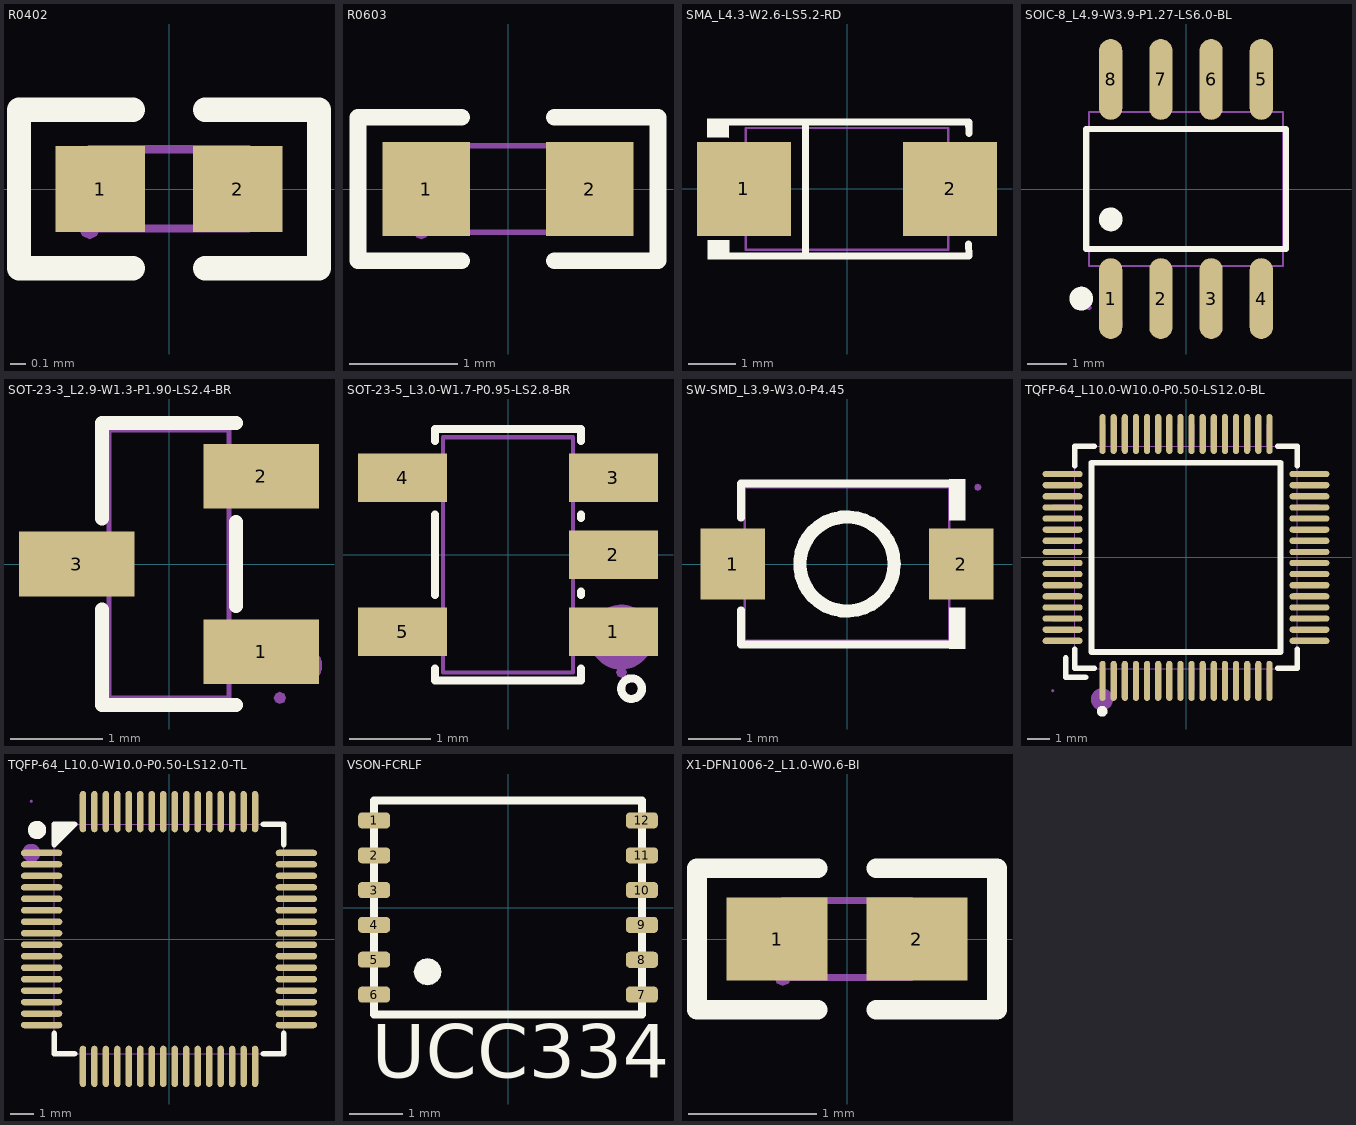
[diagram p0: the footprints below, top view; thin cyan lines are the x and y axes]
# Altium footprint library MISC86293-39.PcbLib: 27 footprints (part 2 of 2)
Each footprint in its own frame and in the unit in brackets; x right, y up, seen from the top. Pads: shape width x height; smd on the part's side, far side on the other; paste and mask are expansions set on the pad; w line width, h text height; cw(c..) or ccw(c..) is an arc to the next point about the centre after c.

## R0402 [mm]
pads (2):
  rect 0.566x0.54 smd paste-100 mask+0.051: 1(-0.433,0) 2(0.433,0)
Top Overlay:
  lines w0.152: -0.226,-0.499 -0.944,-0.499 -0.944,0.499 -0.226,0.499 ; 0.226,-0.499 0.944,-0.499 0.944,0.499 0.226,0.499
Top Paste:
  region: -0.135,-0.23 -0.135,0.23 -0.175,0.27 -0.676,0.27 -0.716,0.23 -0.716,-0.23 -0.676,-0.27 -0.175,-0.27
  region: 0.135,-0.23 0.135,0.23 0.175,0.27 0.676,0.27 0.716,0.23 0.716,-0.23 0.676,-0.27 0.175,-0.27
Mechanical 15:
  region: -0.435,-0.25 -0.454,-0.296 -0.5,-0.315 -0.546,-0.296 -0.565,-0.25 -0.546,-0.204 -0.5,-0.185 -0.454,-0.204
  region: -0.249,0.25 -0.249,-0.25 -0.499,-0.25 -0.499,0.25
  region: 0.251,-0.25 0.251,0.25 0.501,0.25 0.501,-0.25
  lines w0.051: -0.5,-0.25 0.5,-0.25 0.5,0.25 -0.5,0.25 -0.5,-0.25

## R0603 [mm]
pads (2):
  rect 0.806x0.864 smd paste-100 mask+0.051: 1(-0.753,0) 2(0.753,0)
Top Overlay:
  lines w0.152: -0.426,-0.661 -1.385,-0.661 -1.385,0.661 -0.426,0.661 ; 0.426,-0.661 1.385,-0.661 1.385,0.661 0.426,0.661
Top Paste:
  region: -1.195,-0.45 -0.395,-0.45 -0.345,-0.4 -0.345,-0.172 -0.715,-0.172 -0.715,0.158 -0.345,0.158 -0.345,0.4 -0.395,0.45 -1.195,0.45 -1.245,0.4 -1.245,-0.4
  region: 1.195,0.45 0.395,0.45 0.345,0.4 0.345,0.172 0.715,0.172 0.715,-0.158 0.345,-0.158 0.345,-0.4 0.395,-0.45 1.195,-0.45 1.245,-0.4 1.245,0.4
Mechanical 15:
  region: 0.8,-0.4 0.8,0.4 0.5,0.4 0.5,-0.4
  region: -0.8,-0.4 -0.8,0.4 -0.5,0.4 -0.5,-0.4
  region: -0.735,-0.4 -0.754,-0.446 -0.8,-0.465 -0.846,-0.446 -0.865,-0.4 -0.846,-0.354 -0.8,-0.335 -0.754,-0.354
  lines w0.051: -0.8,-0.4 0.8,-0.4 0.8,0.4 -0.8,0.4 -0.8,-0.4

## SMA_L4.3-W2.6-LS5.2-RD [mm]
pads (2):
  rect 2x2 smd: 1(-2.2,0) 2(2.2,0)
Top Overlay:
  region: -2.512,-1.096 -2.513,-1.503 -2.973,-1.498 -2.969,-1.096
  region: -2.52,1.502 -2.521,1.096 -2.981,1.1 -2.977,1.502
  lines w0.152: -2.596,-1.426 2.596,-1.426 ; -2.596,1.426 2.596,1.426 2.603,1.187 ; -0.884,-1.426 -0.884,1.426 ; 2.593,-1.176 2.6,-1.415
Mechanical 6:
  region: 2.014,-0.675 2.014,0.675 1.811,0.675 1.811,-0.675
  region: 2.29,-0.09 2.29,0.112 1.48,0.112 1.48,-0.09
  region: -2.317,-0.101 -2.317,0.101 -1.507,0.101 -1.507,-0.101
Mechanical 15:
  region: -1.48,0.725 -1.48,-0.725 -2.605,-0.725 -2.605,0.725
  region: 2.605,0.725 2.605,-0.725 1.48,-0.725 1.48,0.725
  region: -2.54,-1.3 -2.559,-1.346 -2.605,-1.365 -2.651,-1.346 -2.67,-1.3 -2.651,-1.254 -2.605,-1.235 -2.559,-1.254
  lines w0.051: -2.16,-1.3 2.16,-1.3 2.16,1.3 -2.16,1.3 -2.16,-1.3

## SOIC-8_L4.9-W3.9-P1.27-LS6.0-BL [mm]
pads (8):
  oval 0.588x2.045 smd: 1(-1.905,-2.772) 2(-0.635,-2.772) 3(0.635,-2.772) 4(1.905,-2.772) 5(1.905,2.772) 6(0.635,2.772) 7(-0.635,2.772) 8(-1.905,2.772)
Top Overlay:
  circle w0.3: c-2.652,-2.772 r0.15
  circle w0.3: c-1.905,-0.769 r0.15
  lines w0.152: -2.526,-1.521 2.526,-1.521 2.526,1.521 -2.526,1.521 -2.526,-1.521
Mechanical 6:
  circle w0.3: c-1.905,-3.4 r0.15
Mechanical 15:
  region: 1.695,2.175 1.695,1.94 2.115,1.94 2.115,2.175
  region: 1.695,3 1.695,2.165 2.115,2.165 2.115,3
  region: 0.425,2.175 0.425,1.94 0.845,1.94 0.845,2.175
  region: 0.425,3 0.425,2.165 0.845,2.165 0.845,3
  region: -0.845,2.175 -0.845,1.94 -0.425,1.94 -0.425,2.175
  region: -0.845,3 -0.845,2.165 -0.425,2.165 -0.425,3
  region: -2.115,2.175 -2.115,1.94 -1.695,1.94 -1.695,2.175
  region: -2.115,3 -2.115,2.165 -1.695,2.165 -1.695,3
  region: 1.695,-2.175 1.695,-1.94 2.115,-1.94 2.115,-2.175
  region: 1.695,-3 1.695,-2.165 2.115,-2.165 2.115,-3
  region: 0.425,-2.175 0.425,-1.94 0.845,-1.94 0.845,-2.175
  region: 0.425,-3 0.425,-2.165 0.845,-2.165 0.845,-3
  region: -0.845,-2.175 -0.845,-1.94 -0.425,-1.94 -0.425,-2.175
  region: -0.845,-3 -0.845,-2.165 -0.425,-2.165 -0.425,-3
  region: -2.115,-2.175 -2.115,-1.94 -1.695,-1.94 -1.695,-2.175
  region: -2.115,-3 -2.115,-2.165 -1.695,-2.165 -1.695,-3
  region: -2.385,-3 -2.404,-3.046 -2.45,-3.065 -2.496,-3.046 -2.515,-3 -2.496,-2.954 -2.45,-2.935 -2.404,-2.954
  lines w0.051: -2.45,-1.95 2.45,-1.95 2.45,1.95 -2.45,1.95 -2.45,-1.95

## SOT-23-3_L2.9-W1.3-P1.90-LS2.4-BR [mm]
pads (3):
  rect 1.25x0.7 smd: 1(1,-0.95) 2(1,0.95) 3(-1,0)
Top Overlay:
  lines w0.152: -0.726,-0.495 -0.726,-1.526 0.726,-1.526 ; -0.726,0.495 -0.726,1.526 0.726,1.526 ; 0.726,-0.455 0.726,0.455
Mechanical 6:
  circle w0.2: c1.46,-1.1 r0.1
Mechanical 15:
  region: -1.2,-0.215 -1.2,0.215 -0.9,0.215 -0.9,-0.215
  region: -0.91,-0.215 -0.91,0.215 -0.64,0.215 -0.64,-0.215
  region: 0.9,-1.165 0.9,-0.735 1.2,-0.735 1.2,-1.165
  region: 0.64,-1.165 0.64,-0.735 0.91,-0.735 0.91,-1.165
  region: 0.9,0.735 0.9,1.165 1.2,1.165 1.2,0.735
  region: 0.64,0.735 0.64,1.165 0.91,1.165 0.91,0.735
  region: 1.265,-1.45 1.246,-1.496 1.2,-1.515 1.154,-1.496 1.135,-1.45 1.154,-1.404 1.2,-1.385 1.246,-1.404
  lines w0.051: -0.65,-1.45 0.65,-1.45 0.65,1.45 -0.65,1.45 -0.65,-1.45

## SOT-23-5_L3.0-W1.7-P0.95-LS2.8-BR [mm]
pads (5):
  rect 1.1x0.6 smd: 1(1.3,-0.95) 2(1.3,0) 3(1.3,0.95) 4(-1.3,0.95) 5(-1.3,-0.95)
Top Overlay:
  circle w0.1: c1.524,-1.651 r0.127
  lines w0.1: -0.9,-1.404 -0.9,-1.55 0.9,-1.55 0.9,-1.404 ; -0.9,-0.496 -0.9,0.496 ; -0.9,1.404 -0.9,1.55 0.9,1.55 0.9,1.404 ; 0.9,-0.496 0.9,-0.454 ; 0.9,0.454 0.9,0.496
Mechanical 6:
  circle w0.4: c1.397,-1.016 r0.2
Mechanical 15:
  region: -1.4,-1.15 -1.4,-0.75 -0.95,-0.75 -0.95,-1.15
  region: -0.96,-1.15 -0.96,-0.75 -0.79,-0.75 -0.79,-1.15
  region: -1.4,0.75 -1.4,1.15 -0.95,1.15 -0.95,0.75
  region: -0.96,0.75 -0.96,1.15 -0.79,1.15 -0.79,0.75
  region: 0.95,0.75 0.95,1.15 1.4,1.15 1.4,0.75
  region: 0.79,0.75 0.79,1.15 0.96,1.15 0.96,0.75
  region: 0.95,-0.2 0.95,0.2 1.4,0.2 1.4,-0.2
  region: 0.79,-0.2 0.79,0.2 0.96,0.2 0.96,-0.2
  region: 0.95,-1.15 0.95,-0.75 1.4,-0.75 1.4,-1.15
  region: 0.79,-1.15 0.79,-0.75 0.96,-0.75 0.96,-1.15
  region: 1.465,-1.45 1.446,-1.496 1.4,-1.515 1.354,-1.496 1.335,-1.45 1.354,-1.404 1.4,-1.385 1.446,-1.404
  lines w0.051: -0.8,-1.45 -0.8,1.45 0.8,1.45 0.8,-1.45 -0.8,-1.45

## SW-SMD_L3.9-W3.0-P4.45 [mm]
pads (2):
  rect 1.23x1.36 smd: 1(-2.185,0) 2(2.185,0)
Top Overlay:
  circle w0.254: c0,0 r0.9
  region: 1.95,1.617 1.95,0.832 2.255,0.832 2.255,1.617
  region: 1.95,-1.617 1.95,-0.832 2.255,-0.832 2.255,-1.617
  lines w0.152: -2.026,-0.883 -2.026,-1.541 2.026,-1.541 ; -2.026,0.883 -2.026,1.541 2.026,1.541
Mechanical 15:
  region: -2.5,0.65 -2.5,-0.65 -1.6,-0.65 -1.6,0.65
  region: 2.5,0.65 2.5,-0.65 1.6,-0.65 1.6,0.65
  region: 2.565,1.465 2.546,1.419 2.5,1.4 2.454,1.419 2.435,1.465 2.454,1.511 2.5,1.53 2.546,1.511
  lines w0.051: -1.95,-1.465 -1.95,1.465 1.95,1.465 1.95,-1.465 -1.95,-1.465

## TQFP-64_L10.0-W10.0-P0.50-LS12.0-BL [mm]
pads (64):
  oval 0.28x1.8 smd: 1(-3.75,-5.55) 2(-3.25,-5.55) 3(-2.75,-5.55) 4(-2.25,-5.55) 5(-1.75,-5.55) 6(-1.25,-5.55) 7(-0.75,-5.55) 8(-0.25,-5.55) 9(0.25,-5.55) 10(0.75,-5.55) 11(1.25,-5.55) 12(1.75,-5.55) 13(2.25,-5.55) 14(2.75,-5.55) 15(3.25,-5.55) 16(3.75,-5.55) 33(3.75,5.55) 34(3.25,5.55) 35(2.75,5.55) 36(2.25,5.55) 37(1.75,5.55) 38(1.25,5.55) 39(0.75,5.55) 40(0.25,5.55) 41(-0.25,5.55) 42(-0.75,5.55) 43(-1.25,5.55) 44(-1.75,5.55) 45(-2.25,5.55) 46(-2.75,5.55) 47(-3.25,5.55) 48(-3.75,5.55)
  oval 1.8x0.28 smd: 17(5.55,-3.75) 18(5.55,-3.25) 19(5.55,-2.75) 20(5.55,-2.25) 21(5.55,-1.75) 22(5.55,-1.25) 23(5.55,-0.75) 24(5.55,-0.25) 25(5.55,0.25) 26(5.55,0.75) 27(5.55,1.25) 28(5.55,1.75) 29(5.55,2.25) 30(5.55,2.75) 31(5.55,3.25) 32(5.55,3.75) 49(-5.55,3.75) 50(-5.55,3.25) 51(-5.55,2.75) 52(-5.55,2.25) 53(-5.55,1.75) 54(-5.55,1.25) 55(-5.55,0.75) 56(-5.55,0.25) 57(-5.55,-0.25) 58(-5.55,-0.75) 59(-5.55,-1.25) 60(-5.55,-1.75) 61(-5.55,-2.25) 62(-5.55,-2.75) 63(-5.55,-3.25) 64(-5.55,-3.75)
Top Overlay:
  circle w0.24: c-3.77,-6.92 r0.12
  lines w0.254: -5.4,-4.521 -5.4,-5.39 -4.521,-5.39 ; -5,-4.121 -5,-4.99 -4.121,-4.99 ; -5,4.121 -5,5 -4.121,5 ; 4.121,-4.99 5,-4.99 5,-4.121 ; 4.121,5 5,5 5,4.121 ; -4.25,-4.25 4.25,-4.25 4.25,4.25 -4.25,4.25 -4.25,-4.25
Mechanical 6:
  circle w0.5: c-3.78,-6.38 r0.25
Mechanical 15:
  drawing of 133 lines, arcs and shapes, not listed

## TQFP-64_L10.0-W10.0-P0.50-LS12.0-TL [mm]
pads (64):
  oval 1.8x0.28 smd paste-100 mask+0.051: 1(-5.55,3.75) 2(-5.55,3.25) 3(-5.55,2.75) 4(-5.55,2.25) 5(-5.55,1.75) 6(-5.55,1.25) 7(-5.55,0.75) 8(-5.55,0.25) 9(-5.55,-0.25) 10(-5.55,-0.75) 11(-5.55,-1.25) 12(-5.55,-1.75) 13(-5.55,-2.25) 14(-5.55,-2.75) 15(-5.55,-3.25) 16(-5.55,-3.75) 33(5.55,-3.75) 34(5.55,-3.25) 35(5.55,-2.75) 36(5.55,-2.25) 37(5.55,-1.75) 38(5.55,-1.25) 39(5.55,-0.75) 40(5.55,-0.25) 41(5.55,0.25) 42(5.55,0.75) 43(5.55,1.25) 44(5.55,1.75) 45(5.55,2.25) 46(5.55,2.75) 47(5.55,3.25) 48(5.55,3.75)
  oval 0.28x1.8 smd paste-100 mask+0.051: 17(-3.75,-5.55) 18(-3.25,-5.55) 19(-2.75,-5.55) 20(-2.25,-5.55) 21(-1.75,-5.55) 22(-1.25,-5.55) 23(-0.75,-5.55) 24(-0.25,-5.55) 25(0.25,-5.55) 26(0.75,-5.55) 27(1.25,-5.55) 28(1.75,-5.55) 29(2.25,-5.55) 30(2.75,-5.55) 31(3.25,-5.55) 32(3.75,-5.55) 49(3.75,5.55) 50(3.25,5.55) 51(2.75,5.55) 52(2.25,5.55) 53(1.75,5.55) 54(1.25,5.55) 55(0.75,5.55) 56(0.25,5.55) 57(-0.25,5.55) 58(-0.75,5.55) 59(-1.25,5.55) 60(-1.75,5.55) 61(-2.25,5.55) 62(-2.75,5.55) 63(-3.25,5.55) 64(-3.75,5.55)
Top Overlay:
  circle w0.4: c-5.75,4.75 r0.2
  region: -5,4.25 -5,5 -4.25,5
  lines w0.254: -5,-4.121 -5,-5 -4.121,-5 ; 4.121,-5 5,-5 5,-4.121 ; 4.121,5 5,5 5,4.121 ; -5,4.121 -5,5 -4.121,5 -5,4.121
Top Paste:
  drawing of 64 lines, arcs and shapes, not listed
Mechanical 6:
  circle w0.4: c-6,3.75 r0.2
Mechanical 15:
  drawing of 133 lines, arcs and shapes, not listed

## VSON-FCRLF [mm]
pads (12):
  rrect50% 0.6x0.3 smd: 1(-2.5,1.625) 2(-2.5,0.975) 3(-2.5,0.325) 4(-2.5,-0.323) 5(-2.5,-0.974) 6(-2.5,-1.625) 7(2.5,-1.625) 8(2.5,-0.975) 9(2.5,-0.325) 10(2.5,0.325) 11(2.5,0.975) 12(2.5,1.625)
Top Overlay:
  region: -1.245,-1.2 -1.265,-1.298 -1.32,-1.38 -1.402,-1.435 -1.5,-1.455 -1.598,-1.435 -1.68,-1.38 -1.735,-1.298 -1.755,-1.2 -1.735,-1.102 -1.68,-1.02 -1.598,-0.965 -1.5,-0.945 -1.402,-0.965 -1.32,-1.02 -1.265,-1.102
  lines w0.15: -2.5,-2 -2.5,2 2.5,2 2.5,-2 -2.5,-2
  text "UCC33420" at -2.54,-3.175 h1

## X1-DFN1006-2_L1.0-W0.6-BI [mm]
pads (2):
  rect 0.79x0.648 smd paste-100 mask+0.051: 1(-0.545,0) 2(0.545,0)
Top Overlay:
  lines w0.152: -0.226,-0.553 -1.169,-0.553 -1.169,0.553 -0.226,0.553 ; 0.226,-0.553 1.169,-0.553 1.169,0.553 0.226,0.553
Top Paste:
  region: -0.135,-0.104 -0.135,0.104 -0.404,0.324 -0.892,0.324 -0.94,0.276 -0.94,-0.276 -0.892,-0.324 -0.404,-0.324
  region: 0.135,-0.104 0.135,0.104 0.404,0.324 0.892,0.324 0.94,0.276 0.94,-0.276 0.892,-0.324 0.404,-0.324
Mechanical 15:
  region: 0.5,-0.3 0.5,0.3 0.25,0.3 0.25,-0.3
  region: -0.5,-0.3 -0.5,0.3 -0.25,0.3 -0.25,-0.3
  region: -0.435,-0.3 -0.454,-0.346 -0.5,-0.365 -0.546,-0.346 -0.565,-0.3 -0.546,-0.254 -0.5,-0.235 -0.454,-0.254
  lines w0.051: -0.5,-0.3 0.5,-0.3 0.5,0.3 -0.5,0.3 -0.5,-0.3